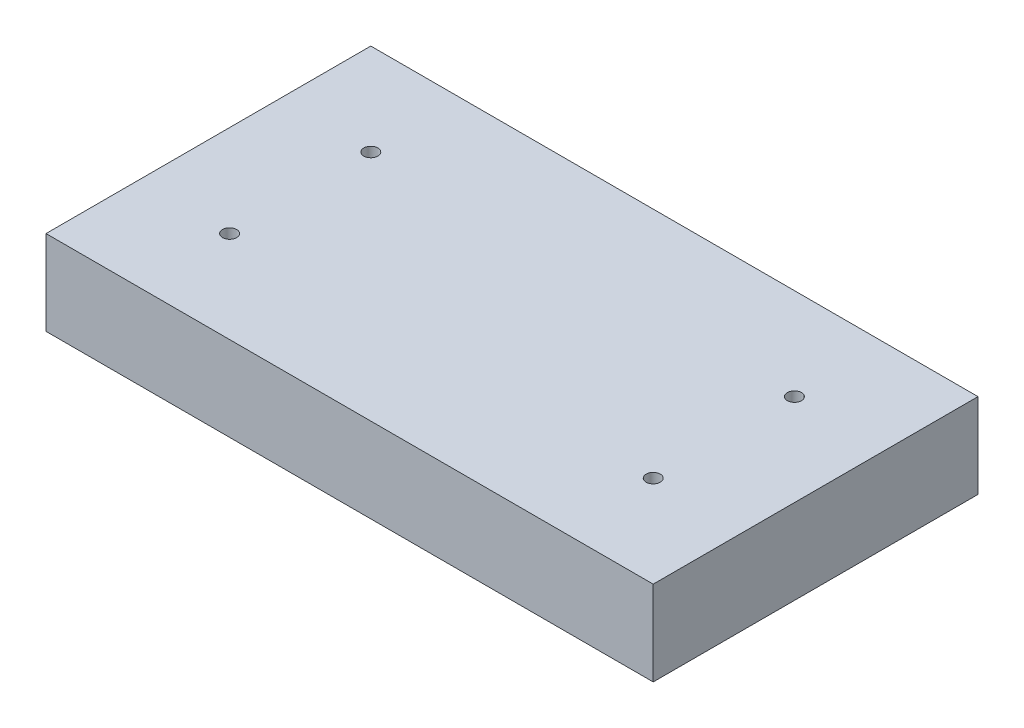
from build123d import *

# Parameters (mm, degrees)
SKETCH_1_W          = 215
SKETCH_1_H          = 115
EXTRUDE_1_DEPTH     = 30
SKETCH_2_R          = 2.5
CUT_EXTRUDE_1_DEPTH = 30


with BuildPart() as part:
    # 草图1 → 凸台-拉伸1 (new body)
    with BuildSketch(Plane(origin=(0, 0, 0), x_dir=(1, 0, 0), z_dir=(0, 1, 0))):
        Rectangle(SKETCH_1_W, SKETCH_1_H)
    extrude(amount=EXTRUDE_1_DEPTH)

    # 草图2 → 切除-拉伸1 (cut)
    with BuildSketch(Plane(origin=(0, 30, 0), x_dir=(1, 0, 0), z_dir=(0, 1, 0))):
        with Locations(Location((-75, 25, 0), (0, 0, 270))):
            Circle(SKETCH_2_R)
        with Locations(Location((75, 25, 0), (0, 0, 270))):
            Circle(SKETCH_2_R)
        with Locations(Location((75, -25, 0), (0, 0, 270))):
            Circle(SKETCH_2_R)
        with Locations(Location((-75, -25, 0), (0, 0, 270))):
            Circle(SKETCH_2_R)
    extrude(amount=-CUT_EXTRUDE_1_DEPTH, mode=Mode.SUBTRACT)


solid = part.part
